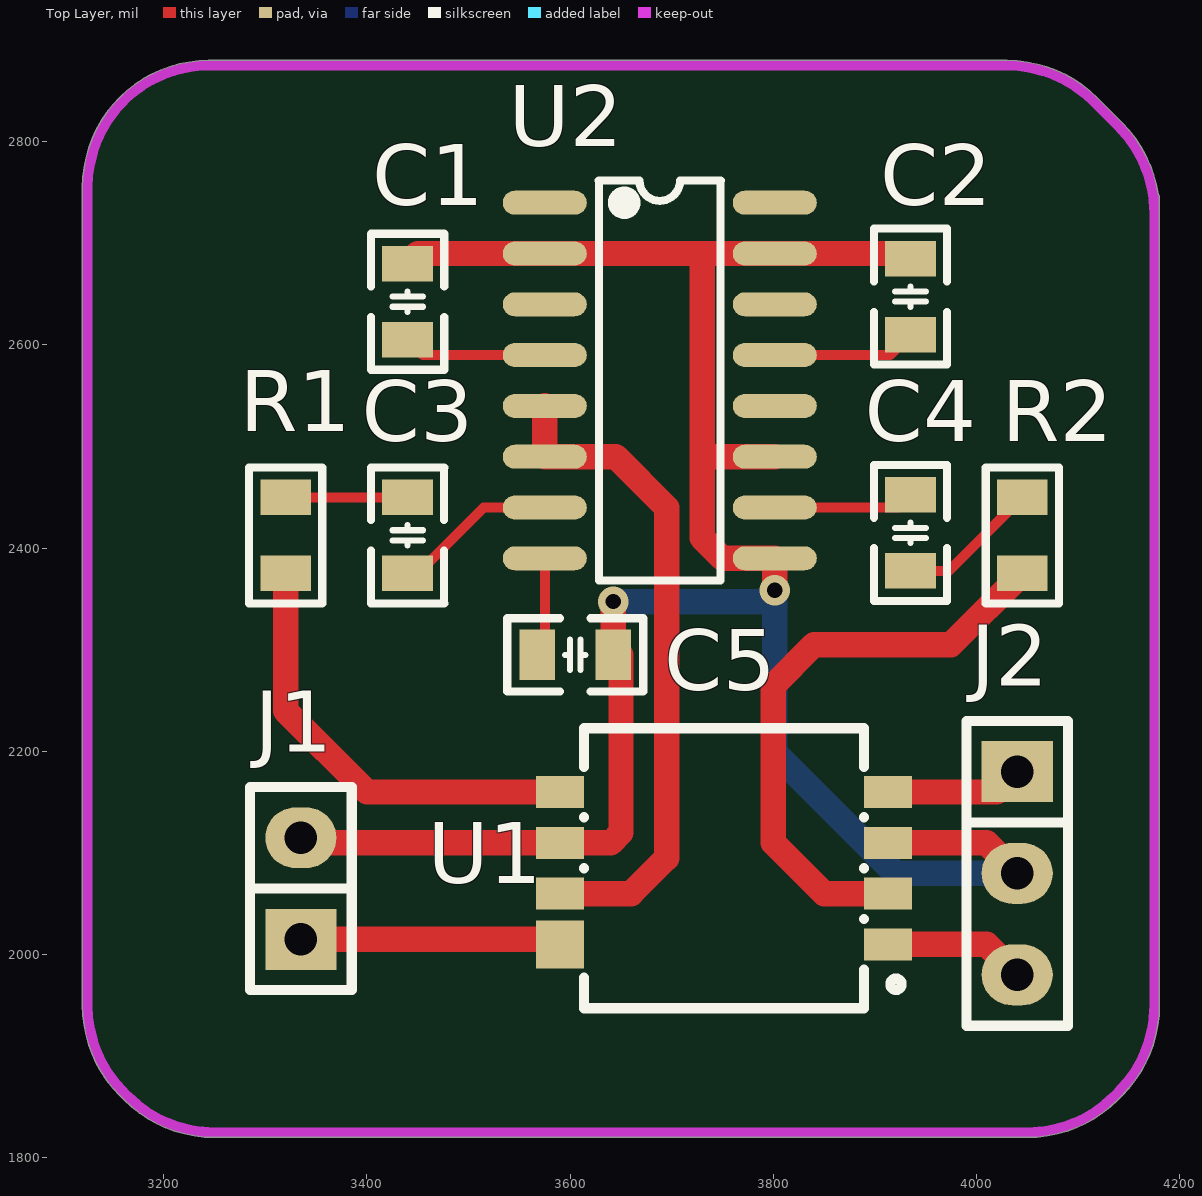
[diagram p0: Top Layer view]
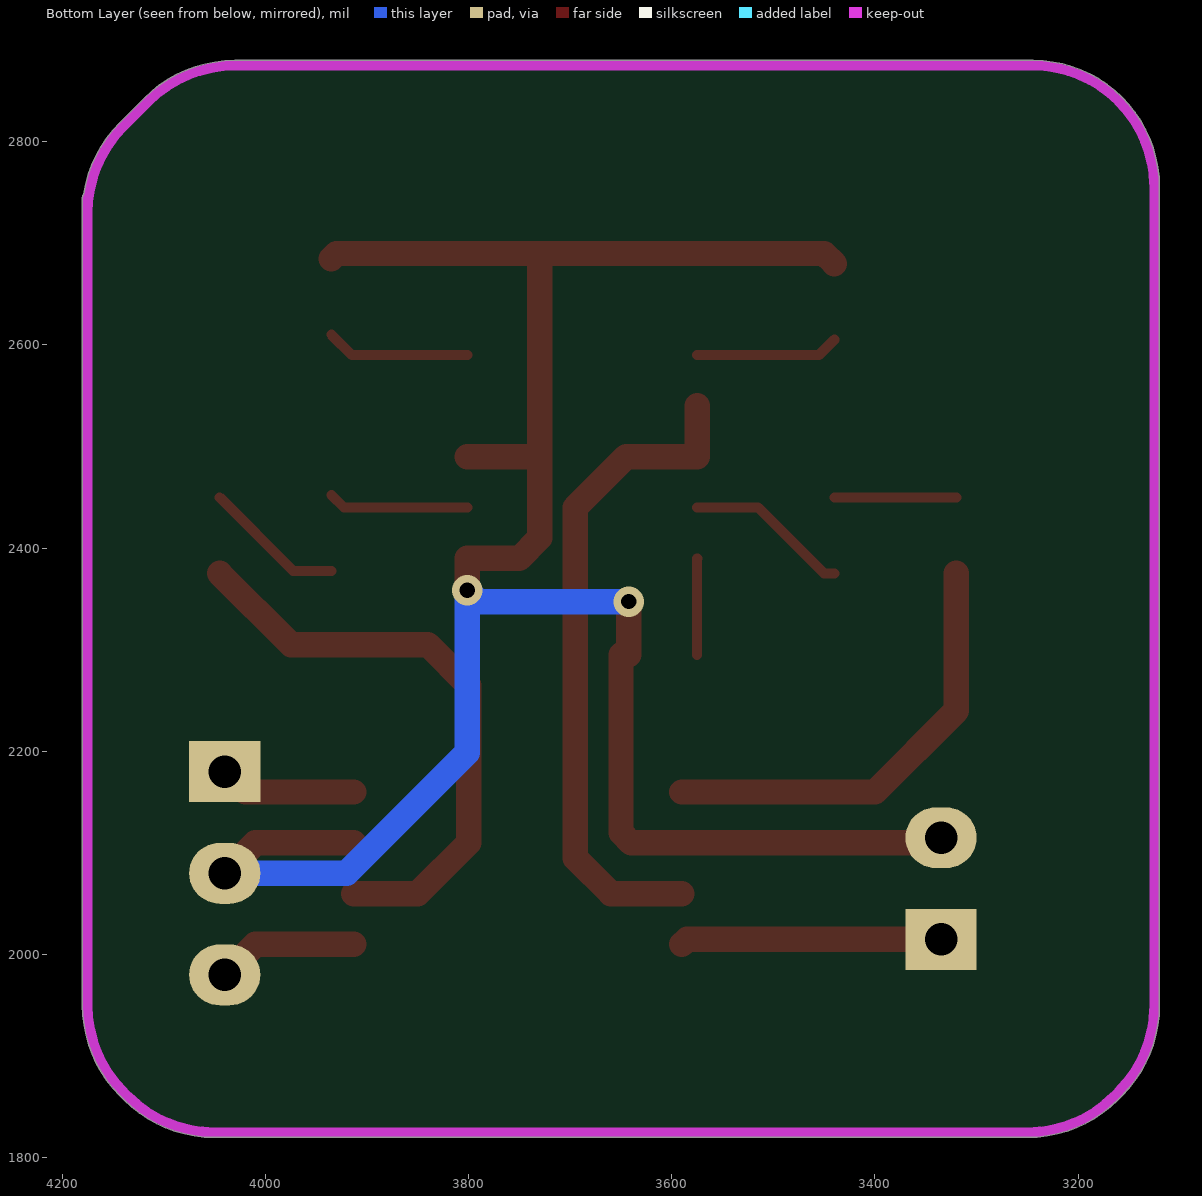
[diagram p1: Bottom Layer view, seen from below]
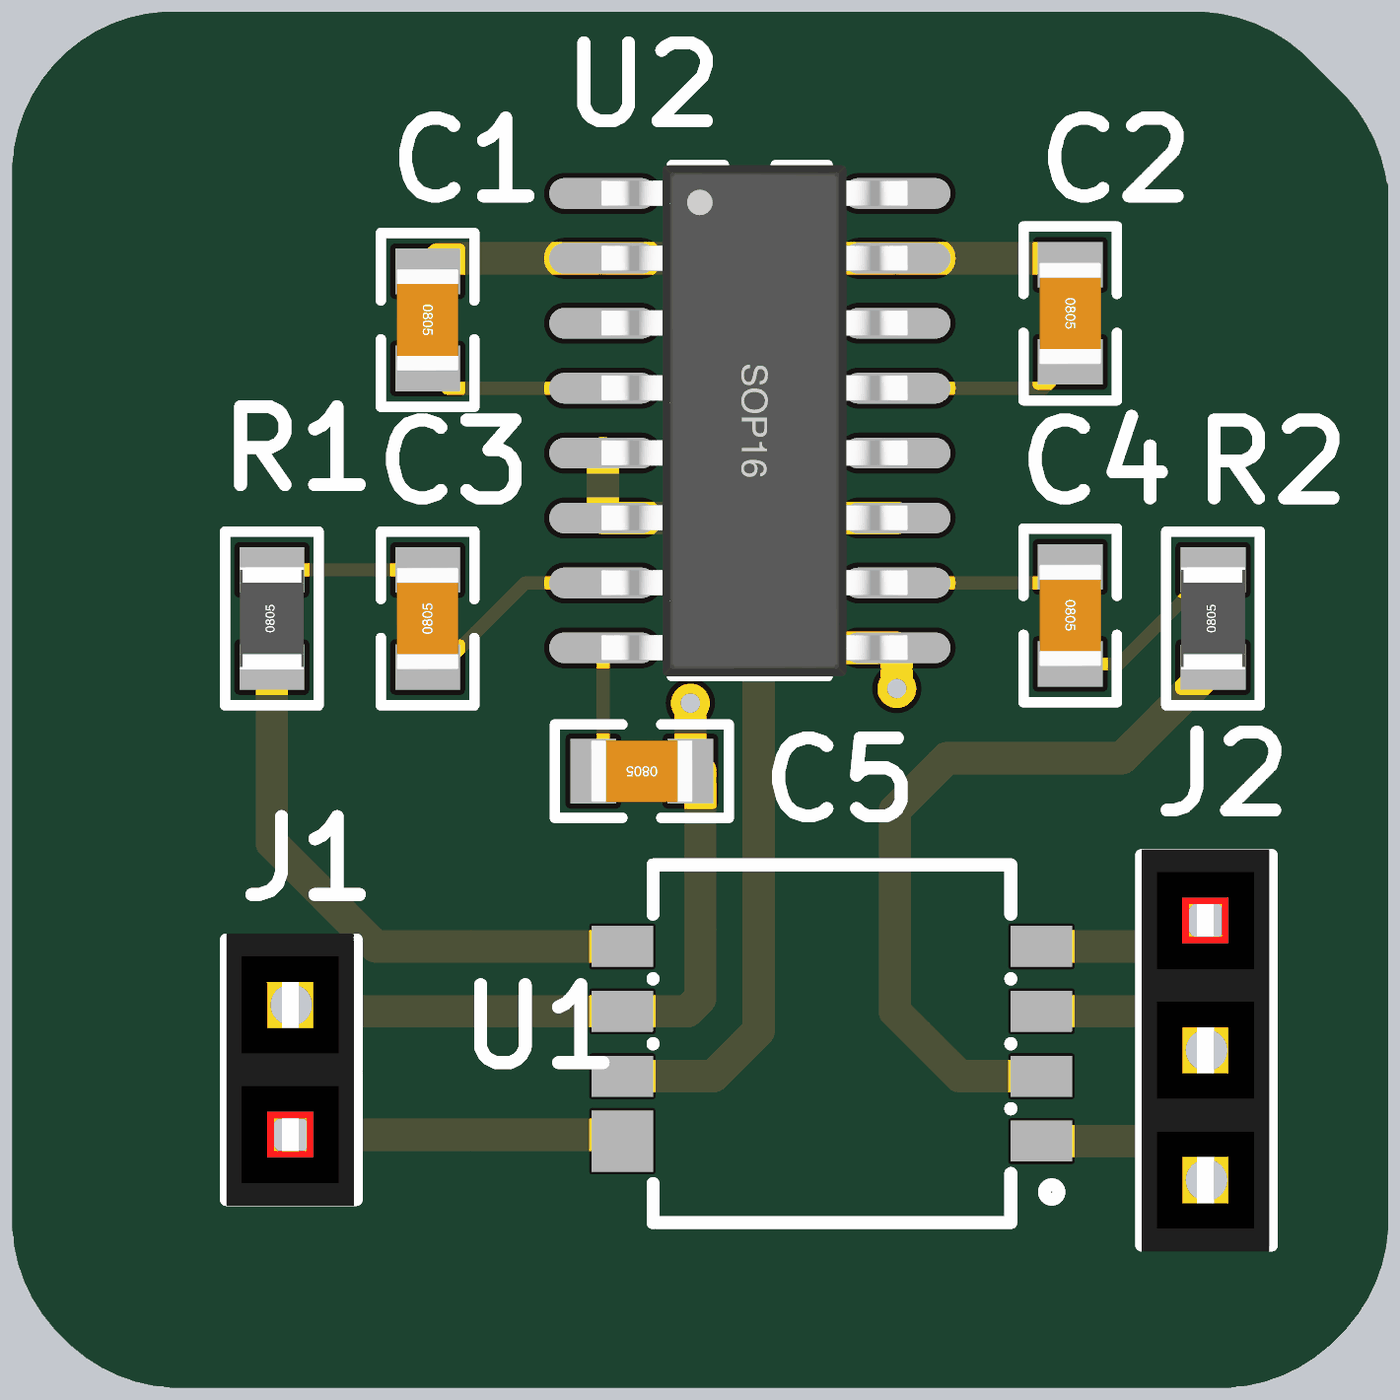
[diagram p2: 3D render of the assembled board from above, using the file's embedded part models]
# Altium PCB MISC84404.PcbDoc
Units mil, origin at the board's own origin, x right, y up, seen from the top; angles counter-clockwise.
Board outline 1060.03 x 1060.03 mil, 2 copper layers (Top Layer, Bottom Layer); 11 components, 14 nets, 43 pads, 2 vias.

## Layer stack, top to bottom (the 12.6 mil dielectric is the usual default, probably not edited)
Top Solder: solder mask 0.4, Solder Resist, Dk 3.5
Top Layer: signal copper 1.4
Dielectric 1: dielectric 12.6, FR-4, Dk 4.8
Bottom Layer: signal copper 1.4
Bottom Solder: solder mask 0.4, Solder Resist, Dk 3.5

## Board outline
3156.81,1861.1 3161.1,1856.81 ccw(c3250,1945.71) 3250,1819.98 4050,1819.98 ccw(c4050,1945.71) 4138.9,1856.81 4143.19,1861.1 ccw(c4054.29,1950) 4180.02,1950 4180.02,2745 ccw(c4175,2745) 4178.66,2748.43 ccw(c4054.29,2730) 4143.19,2818.9 4118.9,2843.19 cw(c4115.36,2839.64) 4118.92,2843.17 4118.9,2843.19 ccw(c4030,2754.29) 4030,2880.01 3243.99,2880.01 ccw(c3243.99,2756.72) 3156.81,2843.9 ccw(c3245.71,2755) 3119.99,2755 3119.99,1950 ccw(c3245.71,1950)

## Design rules (kind name [scope] priority, off if disabled: settings)
Clearance [All] p1: gap=10
MinimumSolderMaskSliver [All] p1: minsoldermaskwidth=0
PolygonConnect [All] p1: connectstyle=Relief reliefconductorwidth=10 reliefentries=4 polygonreliefangle="90 Angle" airgapwidth=10
RoutingVias [All] p1: holewidth=28 width=50 viastyle="Through Hole" minholewidth=28 minwidth=50 maxholewidth=28 maxwidth=50
SilkToSilkClearance [All] p1: silktosilkclearance=0
SilkToSolderMaskClearance [IsPad] p1: minsilkscreentomaskgap=0 clearancetoexposedcopper=TRUE
SolderMaskExpansion [All] p1: expansion=4
Width [All] p1: maxlimit=30 minlimit=10 preferedwidth=10
27 further rules are at their usual default settings.

## Components (designator, comment, footprint, x,y, rotation, side; value= is the part's Value field where it differs from the comment)
C1 "104" "C 0805_L" 3440,2642.6 r270 top
C2 "104" "C 0805_L" 3935,2647.6 r270 top
C3 "104" "C 0805_L" 3440,2412.6 r90 top
C4 "104" "C 0805_L" 3935,2415 r270 top
C5 "104" "C 0805_L" 3605,2295 r180 top
J1 "Female HDR1X2" Fe-HDR1X2/2.54-S 3335,2015 r90 top
J2 "Female HDR1X3" Fe-HDR1X3/2.54-S 4040,2180 r0 top
R1 "103" "R 0805_L" 3320,2412.6 r90 top
R2 "103" "R 0805_L" 4045,2412.6 r90 top
U1 "A50K" SOP-8_L7.0-W7.0-P1.27-LS8.6-BL 3751.42,2085 r90 top
U2 "PAM8406" SOP16 3575,2740 r0 top

## Footprints (in the part's own frame and the unit in brackets; to place one, negate y for a bottom-side part, rotate by r counter-clockwise, add the part's x,y. Pads: shape width x height; smd on the part's side, far side on the other; paste and mask are expansions set on the pad)
"C 0805_L" [mil] "无极性贴片电容"
  rect 35x50 smd: 1(-37.4,0) 2(37.4,0)
  silkscreen extent -67,-36 67,36, body extent -39,-24 39,24, height 20
Fe-HDR1X2/2.54-S [mil] "Connector; Header; 2x2 Position"
  rect 60x70 hole 32: 1(0,0)
  oval 60x70 hole 32: 2(100,0)
  silkscreen extent -50,-50 150,50, body extent -55,-48 155,50, height 335
Fe-HDR1X3/2.54-S [mil]
  rect 70x60 hole 32: 1(0,0)
  oval 70x60 hole 32: 2(0,-100) 3(0,-200)
  silkscreen extent -50,-250 50,50, body extent -50,-255 48,55, height 335
"R 0805_L" [mil] "1/8W贴片电阻"
  rect 35x50 smd: 1(-37.4,0) 2(37.4,0)
  silkscreen extent -67,-36 67,36, body extent -39,-25 39,25, height 20
SOP16 [mm]
  oval 2.1x0.6 smd: 1(0,0) 2(0,-1.27) 3(0,-2.54) 4(0,-3.81) 5(0,-5.08) 6(0,-6.35) 7(0,-7.62) 8(0,-8.89) 9(5.75,-8.89) 10(5.75,-7.62) 11(5.75,-6.35) 12(5.75,-5.08) 13(5.75,-3.81) 14(5.75,-2.54) 15(5.75,-1.27) 16(5.75,0)
  silkscreen extent 1.35,-9.45 4.4,0.56, body extent -0.04,-9.45 5.97,0.56, height 1.9
SOP-8_L7.0-W7.0-P1.27-LS8.6-BL [mm]
  rect 0.8x1.2 smd paste+0 mask+0.051: 1(-1.905,-4.1) 2(-0.635,-4.1) 3(0.635,-4.1) 4(1.905,-4.1) 5(1.905,4.1) 6(0.635,4.1) 7(-0.635,4.1)
  rect 1.2x1.2 smd paste+0 mask+0.051: 8(-1.905,4.1)
  silkscreen extent -3.5,-4.44 3.5,3.5

## Part data
C1 C2 C3 C4 C5: library part C, "Chip capacitor"
R1 R2: library part R, "Chip resistor"
U1: library part GZP6832A010115KPA50KL

## Via types
v1: diameter 30, hole 15, Top Layer to Bottom Layer, 2 vias

## Nets (pads, with @x,y where several pads share a name; then routed paths per layer and width w, separated by ;. In a path a pad name is that pad's centre, name@x,y a point inside that pad or via, vN(x,y) a via of type N, cw(c..) or ccw(c..) an arc to the next point about the centre after c; other vN are vias at no path point)
GND: C1.1 C2.1 C5.1 J1.2 J2.2 U1.3 U1.6 U2.2 U2.9 U2.11 U2.15 | length 2265.3
  Top Layer w25: J1.2 3340,2110 U1.6 3640,2110 3650,2120 C5.1@3650,2295 ; C1.1 3450,2690 U2.2 3730,2690 ; C5.1 v1(3642.4,2347.4) ; v1(3801.38,2358.62) U2.9 3750,2390 3730,2410 3730,2495 ; U2.11 3735,2490 3730,2495 ; U1.3 4010,2110 J2.2 ; C2.1 3930,2690 U2.15 3730,2690 ; 3730,2495 3730,2690
  Bottom Layer w25: v1(3642.4,2347.4) 3790.16,2347.4 v1(3801.38,2358.62) 3801.38,2198.62 3920,2080 J2.2
INL: R1.1 U1.5 | length 438.3
  Top Layer w25: R1.1 3320,2240 3400,2160 U1.5
INR: R2.1 U1.2 | length 579.2
  Top Layer w25: U1.2 3850,2060 3800,2110 3800,2265 3840,2305 3974.8,2305 R2.1
L: J2.1 U1.4 | length 135.5
  Top Layer w25: U1.4 4020,2160 J2.1
NetC1_2: C1.2 U2.4 | length 141.3
  Top Layer w10: C1.2 3455.2,2590 U2.4
NetC2_2: C2.2 U2.13 | length 142
  Top Layer w10: U2.13 3914.8,2590 C2.2
NetC3_1: C3.1 U2.7 | length 161.8
  Top Layer w10: C3.1 3450.2,2375.2 3515,2440 U2.7
NetC3_2: C3.2 R1.2 | length 120
  Top Layer w10: R1.2 C3.2
NetC4_1: C4.1 U2.10 | length 138.8
  Top Layer w10: U2.10 3922.59,2440 C4.1
NetC4_2: C4.2 R2.2 | length 140
  Top Layer w10: C4.2 3972.6,2377.6 R2.2
NetC5_2: C5.2 U2.8 | length 95.1
  Top Layer w10: U2.8 3575.2,2389.8 C5.2@3575.2,2295
NetJ1_1: J1.1 U1.8 | length 257.1
  Top Layer w25: J1.1 3585,2015 U1.8
NetU1_7: U1.7 U2.5 U2.6 | length 655.2
  Top Layer w25: U2.5 U2.6 3645,2490 3695,2440 3695,2095 3660,2060 U1.7
R: J2.3 U1.1 | length 139.6
  Top Layer w25: U1.1 4010,2010 J2.3
pads on no net: U2.1 U2.3 U2.12 U2.14 U2.16

## Keep-outs
Keep-Out Layer:
  lines w10: 3400,2875 4030,2875 cw(c4030,2754.29) 4115.36,2839.64 4139.64,2815.36 cw(c4054.29,2730) 4175,2730 4175,2710 ; 3410,2875 3243.99,2875 ccw(c3243.99,2756.72) 3160.36,2840.36 ccw(c3245.71,2755) 3125,2755 3125,1950 ccw(c3245.71,1950) 3160.36,1864.64 3164.64,1860.36 ccw(c3250,1945.71) 3250,1825 4050,1825 ccw(c4050,1945.71) 4135.36,1860.36 4139.64,1864.64 ccw(c4054.29,1950) 4175,1950 4175,2745